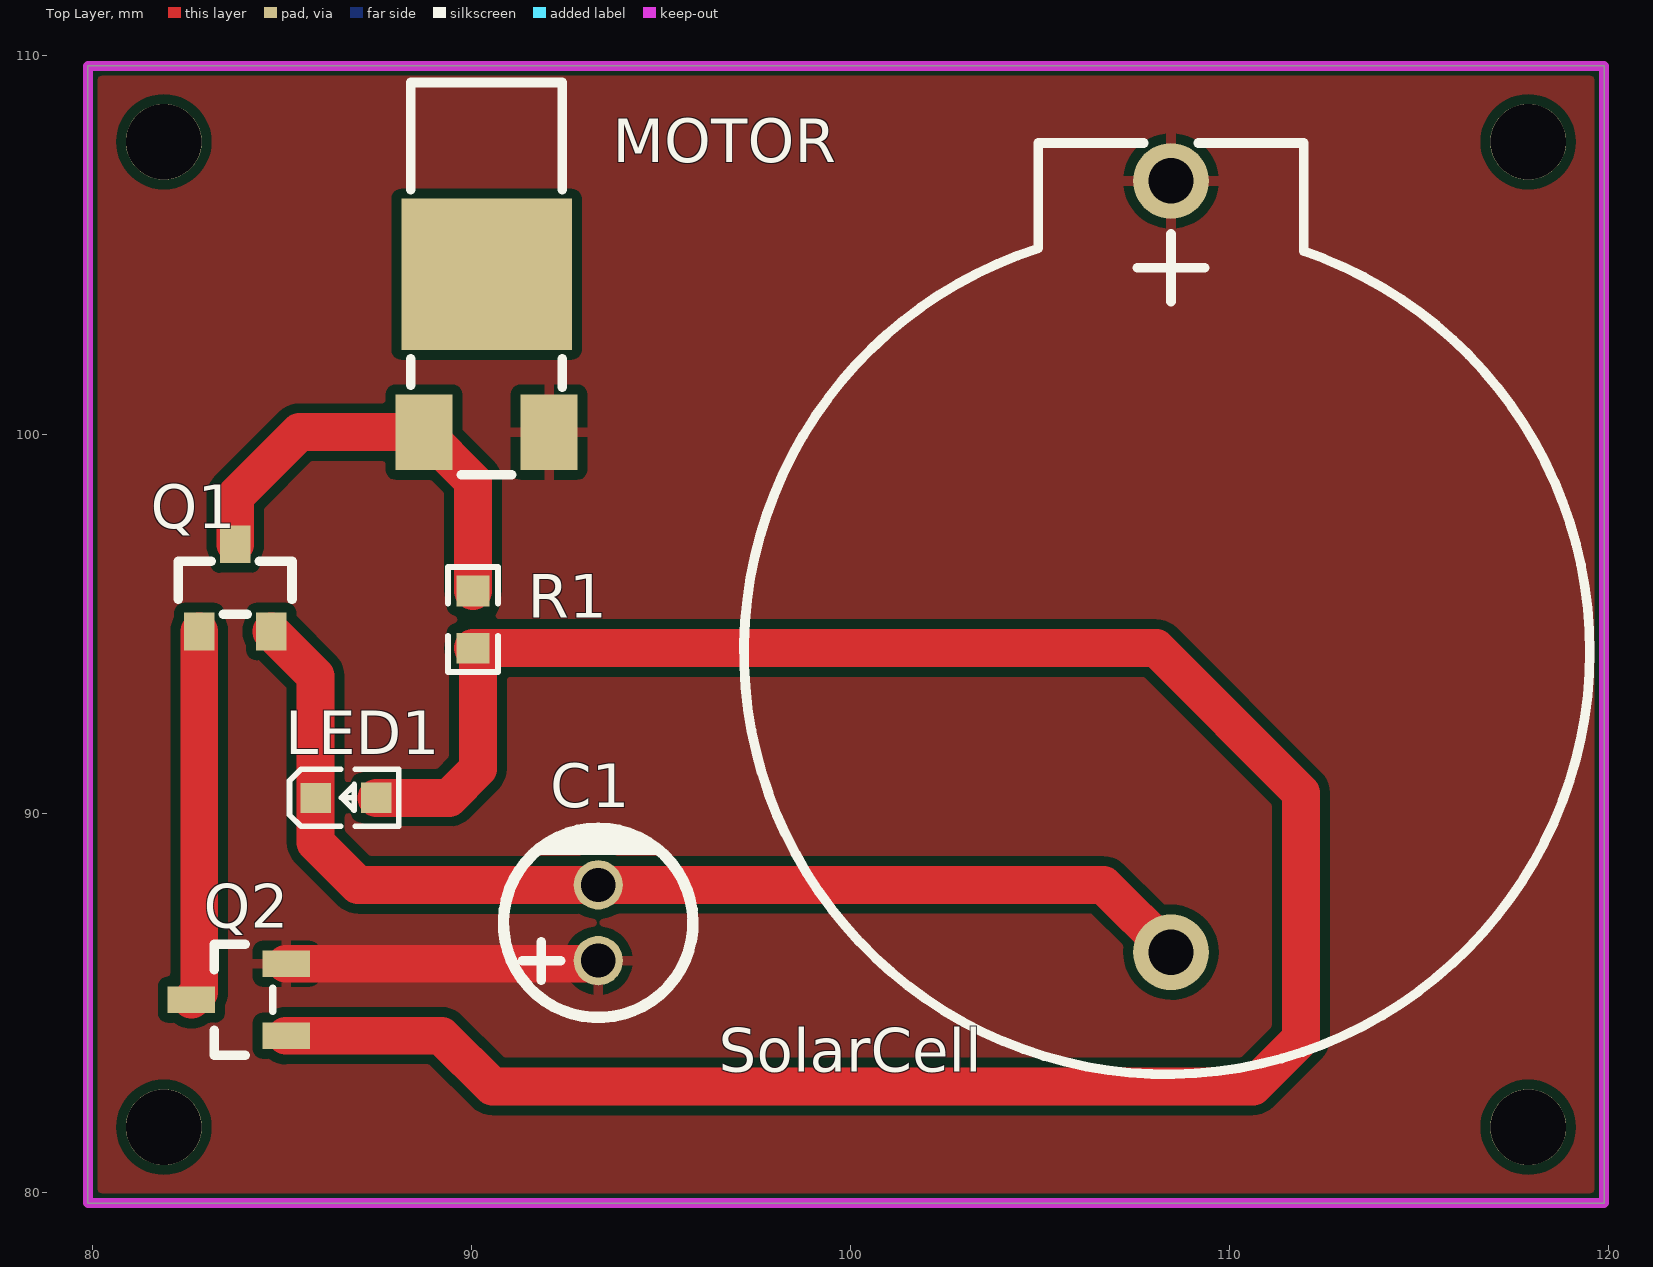
[diagram p0: Top Layer view]
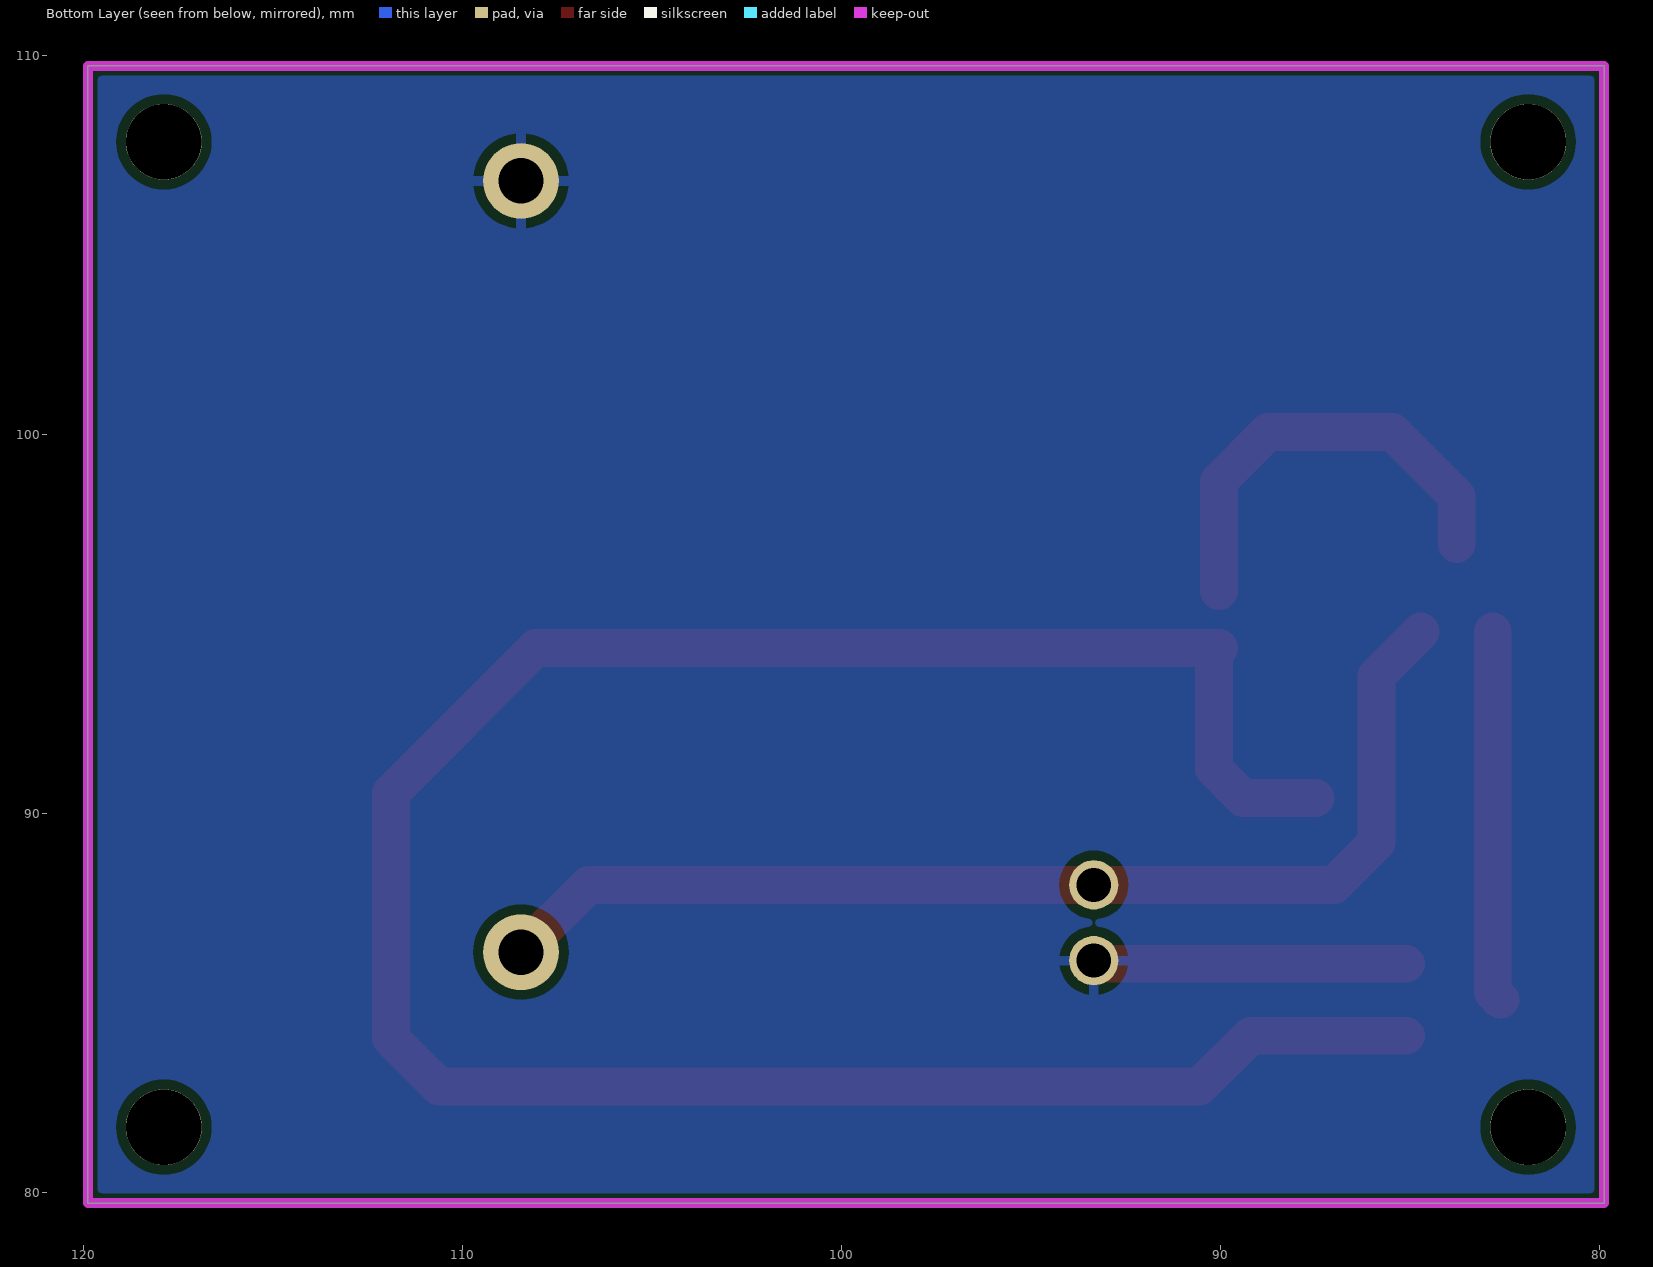
[diagram p1: Bottom Layer view, seen from below]
# Altium PCB MISC49939.pcbdoc
Units mm, origin at the board's own origin, x right, y up, seen from the top; angles counter-clockwise.
Board outline 40 x 30 mm, 2 copper layers (Top Layer, Bottom Layer), stack 1.58 mm thick; 7 components, 5 nets, 21 pads, 0 vias.

## Layer stack, top to bottom
Top Solder Mask Layer: solder mask 0.01, Dk 3.3
Top Layer: signal copper 0.035
Dielectric1: surface 1.51, FR4, Dk 4.5
Bottom Layer: signal copper 0.035
Bottom Solder Mask Layer: solder mask 0.01, Dk 3.3

## Board outline
79.883,109.728 79.883,79.728 119.883,79.728 119.883,109.728

## Design rules (kind name [scope] priority, off if disabled: settings)
BoardOutlineClearance copperThickness2oz_1 [All] p2 off: genericclearance=0.203 ignorepadtopadclearanceinfootprint=FALSE except(0: Arc-SplitContinuation Track-SplitContinuation SMDPad-SplitContinuation THPad-SplitContinuation Via-SplitContinuation Fill-SplitContinuation Region-SplitContinuation Poly-SplitContinuation Text-SplitContinuation Hole-SplitContinuation; 0.152: Arc-CutoutEdge SMDPad-CutoutEdge THPad-CutoutEdge Via-CutoutEdge Fill-CutoutEdge Region-CutoutEdge Text-CutoutEdge; 0.176: Hole-OutlineEdge Hole-CutoutEdge; 0.254: Poly-OutlineEdge Poly-CutoutEdge; 0.3: Arc-OutlineEdge Track-OutlineEdge SMDPad-OutlineEdge THPad-OutlineEdge Via-OutlineEdge Fill-OutlineEdge Region-OutlineEdge Text-OutlineEdge Track-CutoutEdge)
BoardOutlineClearance copperThickness1oz_1 [All] p4: genericclearance=0.102 ignorepadtopadclearanceinfootprint=FALSE except(0: Arc-SplitContinuation Track-SplitContinuation SMDPad-SplitContinuation THPad-SplitContinuation Via-SplitContinuation Fill-SplitContinuation Region-SplitContinuation Poly-SplitContinuation Text-SplitContinuation Hole-SplitContinuation; 0.152: SMDPad-CutoutEdge THPad-CutoutEdge Via-CutoutEdge Fill-CutoutEdge Region-CutoutEdge Text-CutoutEdge; 0.176: Hole-OutlineEdge Hole-CutoutEdge; 0.254: Poly-OutlineEdge Poly-CutoutEdge; 0.3: Arc-OutlineEdge Track-OutlineEdge SMDPad-OutlineEdge THPad-OutlineEdge Via-OutlineEdge Fill-OutlineEdge Region-OutlineEdge Text-OutlineEdge Arc-CutoutEdge Track-CutoutEdge)
Clearance copperThickness2oz [All] p1 off: gap=0.203 ignorepadtopadclearanceinfootprint=FALSE except(0.152: SMDPad-Track SMDPad-SMDPad THPad-Track SMDPad-THPad THPad-THPad Track-Via SMDPad-Via THPad-Via Via-Via Fill-Track Region-Track Fill-SMDPad Region-SMDPad Fill-THPad Region-THPad Fill-Via Region-Via Fill-Fill Fill-Region Region-Region Arc-Track Arc-SMDPad Arc-THPad Arc-Via Fill-Arc Region-Arc Arc-Arc Text-Track SMDPad-Text Text-THPad Text-Via Fill-Text Region-Text Arc-Text Text-Text; 0.176: Hole-Track Hole-SMDPad Hole-THPad Hole-Via Fill-Hole Region-Hole Hole-Arc Hole-Text; 0.254: Poly-Track Poly-SMDPad Poly-THPad Poly-Via Poly-Fill Poly-Region Poly-Poly Poly-Arc Poly-Text Poly-Hole)
Clearance copperThickness1oz [All] p3: gap=0.102 ignorepadtopadclearanceinfootprint=FALSE except(0.152: SMDPad-Track SMDPad-SMDPad THPad-Track SMDPad-THPad THPad-THPad Track-Via SMDPad-Via THPad-Via Via-Via Fill-Track Region-Track Fill-SMDPad Region-SMDPad Fill-THPad Region-THPad Fill-Via Region-Via Fill-Fill Fill-Region Region-Region Arc-Track Arc-SMDPad Arc-THPad Arc-Via Fill-Arc Region-Arc Arc-Arc Text-Track SMDPad-Text Text-THPad Text-Via Fill-Text Region-Text Arc-Text Text-Text; 0.176: Hole-Track Hole-SMDPad Hole-THPad Hole-Via Fill-Hole Region-Hole Hole-Arc Hole-Text; 0.254: Poly-Track Poly-SMDPad Poly-THPad Poly-Via Poly-Fill Poly-Region Poly-Poly Poly-Arc Poly-Text Poly-Hole)
Creepage creepage [All] p1: checkdistance=0 ignoreinternallayers=TRUE applytopolygonpour=TRUE
DiffPairsRouting differentialPair [All] p1: maxlimit=0.152 minlimit=0.152 mostfreqgap=0.152 toplayer_minwidth=0.127 toplayer_prefwidth=0.254 toplayer_maxwidth=2.54 toplayer_mingap=0.152 toplayer_prefgap=0.152 toplayer_maxgap=0.152 bottomlayer_minwidth=0.127 bottomlayer_prefwidth=0.254 bottomlayer_maxwidth=2.54 bottomlayer_mingap=0.152 bottomlayer_prefgap=0.152 bottomlayer_maxgap=0.152 maxuncoupledlength=0.254
HoleToHoleClearance otherClearance [All] p1: gap=0.3 allowstackedmicrovias=TRUE
Length netLength [All] p1: minlimit=0 maxlimit=0
MatchedLengths netLengthTolerance [All] p1: tolerance=25.4
PasteMaskExpansion pasteMaskExpansion [All] p1: expansion=0
PlaneConnect innerPlane [All] p1: planeconnectstyle=Relief reliefexpansion=0.508 reliefentries=4 reliefconductorwidth=0.254 reliefairgap=0.254
PolygonConnect copperRegion [(InNet('$1N1'))] p1: connectstyle=Relief reliefconductorwidth=0.254 reliefentries=4 polygonreliefangle="90 Angle" airgapwidth=0.254 via.connectstyle=Relief via.reliefconductorwidth=0.254 via.reliefentries=4 via.polygonreliefangle="90 Angle" via.airgapwidth=0.254
RoutingVias viaSize [All] p1: holewidth=0.305 width=0.61 viastyle="Through Hole" minholewidth=0.3 minwidth=0.5 maxholewidth=6.3 maxwidth=10
SolderMaskExpansion solderMaskExpansion [IsVia] p1: expansion=-25.4 istentingtop=TRUE
SolderMaskExpansion solderMaskExpansion [All] p2: expansion=0.051 istentingtop=FALSE
Width copperThickness2oz_2 [All] p1 off: maxlimit=2.54 minlimit=0.203 preferedwidth=0.254
Width copperThickness1oz_2 [All] p2: maxlimit=2.54 minlimit=0.127 preferedwidth=0.254

## Components (designator, comment, footprint, x,y, rotation, side; value= is the part's Value field where it differs from the comment)
C1 "4700uF" CAP-TH_BD5.0-P2.00-D0.8-FD-10UF50VC110GL 93.345,87.122 r90 top
LED1 "" LED_0603 86.741,90.424 r0 top
MOTOR "MOTOR_3" VIBRATING-MOTOR-SMD_3P_C9900012555 90.399,102.15 r270 top
Q1 "" S8050_SOT-23 83.767,95.959 r270 top
Q2 "" S8550P_SOT 83.82,85.09 r0 top
R1 "2.2K" R0603 90.043,95.123 r90 top
SolarCell "1.5V*2" BAT-TH_CR2032-2-1 108.458,96.52 r90 top

## Footprints (in the part's own frame and the unit in brackets; to place one, negate y for a bottom-side part, rotate by r counter-clockwise, add the part's x,y. Pads: shape width x height; smd on the part's side, far side on the other; paste and mask are expansions set on the pad)
BAT-TH_CR2032-2-1 [mm]
  round 2 hole 1.2: 1(10.175,0) 2(-10.175,0)
  silkscreen extent -13.4,-11.05 11.17,11.26
CAP-TH_BD5.0-P2.00-D0.8-FD-10UF50VC110GL [mm]
  round 1.3 hole 0.9 paste+0 mask+0.051: 1(-1,0) 2(1,0)
  silkscreen extent -2.5,-2.5 2.5,2.5
LED_0603 [mil]
  rect 31.5x31.5 smd paste+0 mask+2: 1(-33.5,-0.4) 2(29.5,-0.2)
  silkscreen extent -61,-30 53,30
R0603 [mm]
  rect 0.806x0.864 smd paste-100 mask+0.051: 1(-0.753,0) 2(0.753,0)
  silkscreen extent -1.39,-0.66 1.39,0.66
S8050_SOT-23 [mm]
  rect 1x0.8 smd paste+0 mask+0.051: 1(1.15,-0.95) 2(1.15,0.95) 3(-1.15,0)
  silkscreen extent -0.7,-1.5 0.7,1.5
S8550P_SOT [mm]
  rect 1.25x0.701 smd paste+0 mask+0.051: 1(1.291,-0.95) 2(1.291,0.95) 3(-1.208,0)
  silkscreen extent -0.61,-1.46 0.94,1.46
VIBRATING-MOTOR-SMD_3P_C9900012555 [mm]
  rect 2x1.5 smd paste+0 mask+0.05: 1(2.083,1.65) 2(2.083,-1.65)
  rect 4x4.5 smd paste+0 mask+0.05: 3(-2.084,0)
  silkscreen extent -7.14,-2 3.21,2

## Free pads (board coordinates)
  round 2 hole 2: 1(81.883,81.728) 1(81.883,107.728) 1(117.883,81.728) 1(117.883,107.728)

## Nets (pads, with @x,y where several pads share a name; then routed paths per layer and width w, separated by ;. In a path a pad name is that pad's centre, name@x,y a point inside that pad or via, vN(x,y) a via of type N, cw(c..) or ccw(c..) an arc to the next point about the centre after c; other vN are vias at no path point)
$1N1: C1.1 MOTOR.1 Q2.2 SolarCell.1 | length 8.3
  Top Layer w1: Q2.2 93.263,86.04 C1.1
$1N2: C1.2 LED1.1 Q1.2 SolarCell.2 | length 29.8
  Top Layer w1: Q1.2 85.89,93.637 LED1.1 85.89,89.243 87.011,88.122 C1.2 106.681,88.122 SolarCell.2
$1N3: Q1.1 Q2.3 | length 9.8
  Top Layer w1: Q2.3 82.817,85.295 Q1.1
$1N4: MOTOR.2 Q1.3 R1.2 | length 11.7
  Top Layer w1: Q1.3 83.767,98.372 85.461,100.066 MOTOR.2 90.043,98.772 R1.2
$1N5: LED1.2 Q2.1 R1.1 | length 64
  Top Layer w1: Q2.1 89.215,84.14 90.551,82.804 110.617,82.804 111.887,84.074 111.887,90.551 108.068,94.37 R1.1 90.17,94.243 90.17,91.186 89.403,90.419 LED1.2
pads on no net: MOTOR.3

## Polygon pours and split planes (outlines as drawn)
$1N1 on Top Layer (solid, remove dead copper, pour order 0): 76.2,112.395 76.2,76.2 124.968,76.2 124.968,112.395
$1N1 on Bottom Layer (solid, remove dead copper, pour order 2): 76.962,112.522 76.962,77.343 123.19,77.343 123.19,112.522

## Keep-outs
Board Outline Layer:
  the board outline again, w0.254